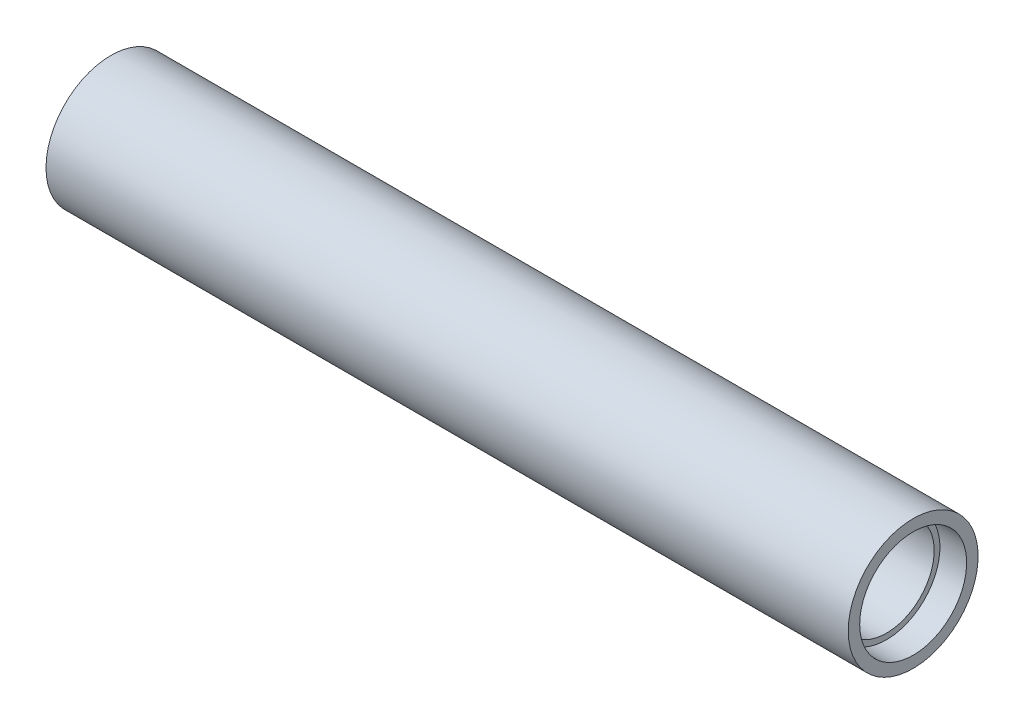
from build123d import *


with BuildPart() as part:
    # 草图1 → 旋转1 (revolve)
    with BuildSketch(Plane.XY, mode=Mode.PRIVATE) as revolve_1_sk:
        Polygon((105, 17), (-105, 17), (-105, 14), (-98, 14), (-98, 12.5), (98, 12.5), (98, 14), (105, 14), align=None)
    revolve(revolve_1_sk.sketch.rotate(Axis((0, 0, 0), (1, 0, 0)), 90), axis=Axis((0, 0, 0), (1, 0, 0)))


solid = part.part
